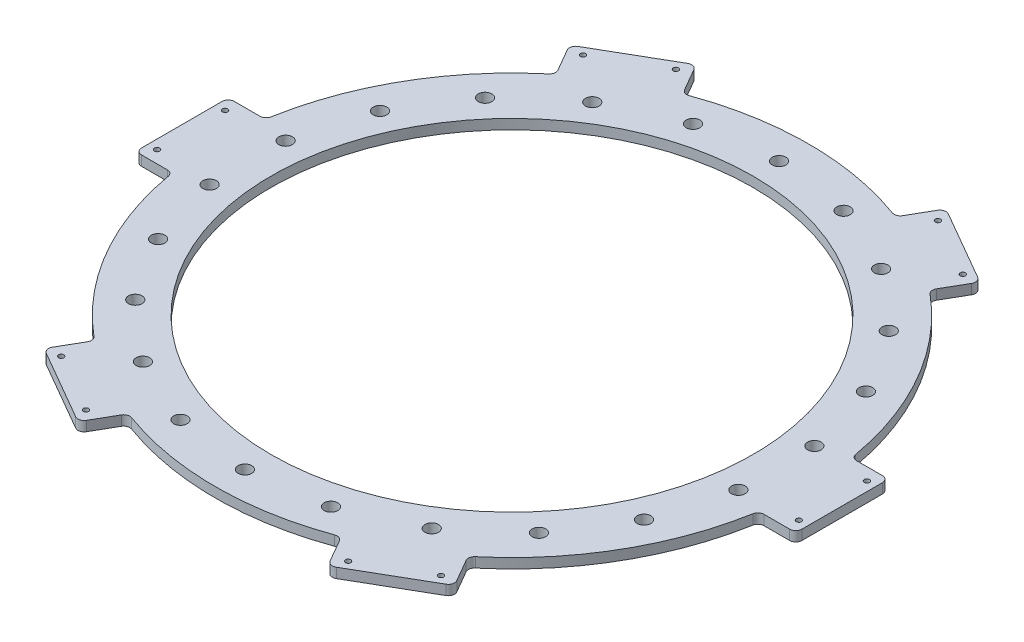
SolidWorks part; units mm, degrees
material "Q235B"
ref_plane "Front Plane" through (0, 0, 0) normal (0, 0, 1) x (1, 0, 0)
ref_plane "Top Plane" through (0, 0, 0) normal (0, 1, 0) x (1, 0, 0)
ref_plane "Right Plane" through (0, 0, 0) normal (1, 0, 0) x (0, 0, -1)
sketch "Sketch2" plane through (0, 0, 0) normal (0, 1, 0) x (1, 0, 0)
  line L0 (-474.1044, 75) -> (-524, 75)
  line L1 (-534, 65) -> (-534, -65)
  line L2 (-534, 0) -> (-480, 0) construction
  line L3 (-474.1044, -75) -> (-524, -75)
  line L4 (0, 0) -> (0, 390) construction
  line L5 (-172.1003, 448.0865) -> (-197.0481, 491.2973)
  line L6 (-210.7083, 494.9576) -> (-323.2917, 429.9576)
  line L7 (-302.0041, 373.0865) -> (-326.9519, 416.2973)
  line L8 (-267, 462.4576) -> (-240, 415.6922) construction
  line L9 (302.0041, 373.0865) -> (326.9519, 416.2973)
  line L10 (323.2917, 429.9576) -> (210.7083, 494.9576)
  line L11 (172.1003, 448.0865) -> (197.0481, 491.2973)
  line L12 (267, 462.4576) -> (240, 415.6922) construction
  line L13 (474.1044, -75) -> (524, -75)
  line L14 (534, -65) -> (534, 65)
  line L15 (474.1044, 75) -> (524, 75)
  line L16 (534, 0) -> (480, 0) construction
  line L17 (172.1003, -448.0865) -> (197.0481, -491.2973)
  line L18 (210.7083, -494.9576) -> (323.2917, -429.9576)
  line L19 (302.0041, -373.0865) -> (326.9519, -416.2973)
  line L20 (267, -462.4576) -> (240, -415.6922) construction
  line L21 (-302.0041, -373.0865) -> (-326.9519, -416.2973)
  line L22 (-323.2917, -429.9576) -> (-210.7083, -494.9576)
  line L23 (-172.1003, -448.0865) -> (-197.0481, -491.2973)
  line L24 (-267, -462.4576) -> (-240, -415.6922) construction
  circle A0 centre (0, 0) radius 390
  circle A1 centre (0, 0) radius 480
  arc A3 (-524, -75) -> (-534, -65) centre (-524, -65) cw
  arc A4 (-524, 75) -> (-534, 65) centre (-524, 65) ccw
  arc A5 (-326.9519, 416.2973) -> (-323.2917, 429.9576) centre (-318.2917, 421.2973) cw
  arc A6 (-197.0481, 491.2973) -> (-210.7083, 494.9576) centre (-205.7083, 486.2973) ccw
  arc A7 (197.0481, 491.2973) -> (210.7083, 494.9576) centre (205.7083, 486.2973) cw
  arc A8 (326.9519, 416.2973) -> (323.2917, 429.9576) centre (318.2917, 421.2973) ccw
  arc A9 (524, 75) -> (534, 65) centre (524, 65) cw
  arc A10 (524, -75) -> (534, -65) centre (524, -65) ccw
  arc A11 (326.9519, -416.2973) -> (323.2917, -429.9576) centre (318.2917, -421.2973) cw
  arc A12 (197.0481, -491.2973) -> (210.7083, -494.9576) centre (205.7083, -486.2973) ccw
  arc A13 (-197.0481, -491.2973) -> (-210.7083, -494.9576) centre (-205.7083, -486.2973) cw
  arc A14 (-326.9519, -416.2973) -> (-323.2917, -429.9576) centre (-318.2917, -421.2973) ccw
  point P15 (-534, -75)
  point P18 (-534, 75)
  point P71 (0, 0)
  dimension "D1" = 780
  dimension "D2" = 960
  dimension "D6" = 10
  dimension "D4" = 1068
  dimension "D5" = 150
  dimension "D7" = 6
extrude "Boss-Extrude1" add sketch "Sketch2" along normal blind 16 contours A1 A0 | L5 A6 L6 A5 L7 A1 | L0 A4 L1 A3 L3 A1 | L21 A14 L22 A13 L23 A1 | L17 A12 L18 A11 L19 A1 | L13 A10 L14 A9 L15 A1 | L9 A8 L10 A7 L11 A1
fillet "Fillet1" radius 10 12 edges at (-302.0041, 8, -373.0865) (-172.1003, 8, -448.0865) (172.1003, 8, -448.0865) (302.0041, 8, -373.0865) (474.1044, 8, -75) (474.1044, 8, 75) (302.0041, 8, 373.0865) (172.1003, 8, 448.0865) (-172.1003, 8, 448.0865) (-302.0041, 8, 373.0865) (-474.1044, 8, 75) (-474.1044, 8, -75)
hole_wizard "Ø22.0 (22) Diameter Hole1" positions "Sketch3" profile "Sketch4" hole size "Ø22.0" standard "GB" end condition up to next
sketch "Sketch3" plane through (0, 16, 0) normal (0, 1, 0) x (1, 0, 0)
  circle A0 centre (0, 0) radius 432 construction
  point P0 (0, 432)
  point P13 (121.7085, 414.501)
  point P14 (233.5568, 363.4215)
  point P15 (326.4838, 282.8998)
  point P16 (392.961, 179.4593)
  point P17 (427.6029, 61.48)
  point P18 (427.6029, -61.48)
  point P19 (392.961, -179.4593)
  point P20 (326.4838, -282.8998)
  point P21 (233.5568, -363.4215)
  point P22 (121.7085, -414.501)
  point P23 (0, -432)
  point P24 (-121.7085, -414.501)
  point P25 (-233.5568, -363.4215)
  point P26 (-326.4838, -282.8998)
  point P27 (-392.961, -179.4593)
  point P28 (-427.6029, -61.48)
  point P29 (-427.6029, 61.48)
  point P30 (-392.961, 179.4593)
  point P31 (-326.4838, 282.8998)
  point P32 (-233.5568, 363.4215)
  point P33 (-121.7085, 414.501)
  dimension "D1" = 864
  dimension "D2" = 22
sketch "Sketch4" plane through (0, 16, -432) normal (1, 0, 0) x (0, 0, 1)
  line L0 (0, 0) -> (0, 16)
  line L1 (0, 16) -> (11, 16)
  line L2 (11, 16) -> (11, 0)
  line L5 (11, 0) -> (0, 0)
  line L11 (0, -6.35) -> (0, 107.95) construction
  dimension "通孔孔直径" = 22
  dimension "通孔孔深度" = 16
hole_wizard "M10 Tapped Hole1" positions "Sketch5" profile "Sketch6" tap size "M10" standard "GB" end condition up to next
sketch "Sketch5" plane through (0, 16, 0) normal (0, 1, 0) x (1, 0, 0)
  line L0 (0, 0) -> (-727.0672, 0) construction
  circle A0 centre (0, 0) radius 522 construction
  point P0 (-519.0944, 55)
  point P2 (-519.0944, -55)
  point P17 (-211.9158, 477.0489)
  point P18 (-307.1786, 422.0489)
  point P19 (307.1786, 422.0489)
  point P20 (211.9158, 477.0489)
  point P21 (519.0944, -55)
  point P22 (519.0944, 55)
  point P23 (211.9158, -477.0489)
  point P24 (307.1786, -422.0489)
  point P25 (-307.1786, -422.0489)
  point P26 (-211.9158, -477.0489)
  dimension "D1" = 1044
  dimension "D2" = 110
  dimension "D3" = 6
sketch "Sketch6" plane through (-519.0944, 16, -55) normal (1, 0, 0) x (0, 0, 1)
  line L0 (0, 0) -> (0, 16)
  line L1 (0, 16) -> (4.25, 16)
  line L2 (4.25, 16) -> (4.25, 0)
  line L5 (4.25, 0) -> (0, 0)
  line L11 (0, -6.35) -> (0, 107.95) construction
  dimension "通孔螺纹孔钻头直径" = 8.5
  dimension "通孔螺纹孔钻头深度" = 16
cosmetic thread "CosmeticThread1" parameters "D2"=10
cosmetic thread "CosmeticThread2" parameters "D2"=10
cosmetic thread "CosmeticThread3" parameters "D2"=10
cosmetic thread "CosmeticThread4" parameters "D2"=10
cosmetic thread "CosmeticThread5" parameters "D2"=10
cosmetic thread "CosmeticThread6" parameters "D2"=10
cosmetic thread "CosmeticThread7" parameters "D2"=10
cosmetic thread "CosmeticThread8" parameters "D2"=10
cosmetic thread "CosmeticThread9" parameters "D2"=10
cosmetic thread "CosmeticThread10" parameters "D2"=10
cosmetic thread "CosmeticThread11" parameters "D2"=10
cosmetic thread "CosmeticThread12" parameters "D2"=10
sketch "Sketch7" plane through (0, 0, 0) normal (0, 1, 0) x (1, 0, 0)
  circle A0 centre (0, 0) radius 538 construction
  dimension "D1" = 1076
